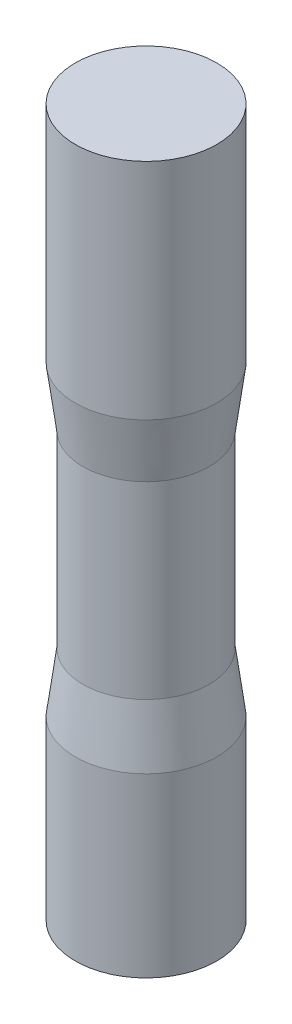
SolidWorks part; units mm, degrees
ref_plane "Front Plane" through (0, 0, 0) normal (0, 0, 1) x (1, 0, 0)
ref_plane "Top Plane" through (0, 0, 0) normal (0, 1, 0) x (1, 0, 0)
ref_plane "Right Plane" through (0, 0, 0) normal (1, 0, 0) x (0, 0, -1)
sketch "Sketch1" plane through (0, 0, 0) normal (0, 0, 1) x (1, 0, 0)
  line L0 (0, 0) -> (-3, 0)
  line L1 (-3, 0) -> (-3, -9.5)
  line L2 (-3, -9.5) -> (-2.675, -12)
  line L3 (-2.675, -12) -> (-2.675, -20)
  line L4 (-2.675, -20) -> (-3, -22.5)
  line L5 (-3, -22.5) -> (-3, -30)
  line L6 (-3, -30) -> (0, -30)
  line L7 (0, -30) -> (0, 0)
  dimension "D1" = 12
  dimension "D2" = 2.5
  dimension "D3" = 18
  dimension "D4" = 10
  dimension "D5" = 2.5
  dimension "D6" = 3
  dimension "D7" = 2.675
revolve "Revolve1" add sketch "Sketch1" angle 360 about L7
cosmetic thread "Cosmetic Thread1" parameters "D2"=4.917
